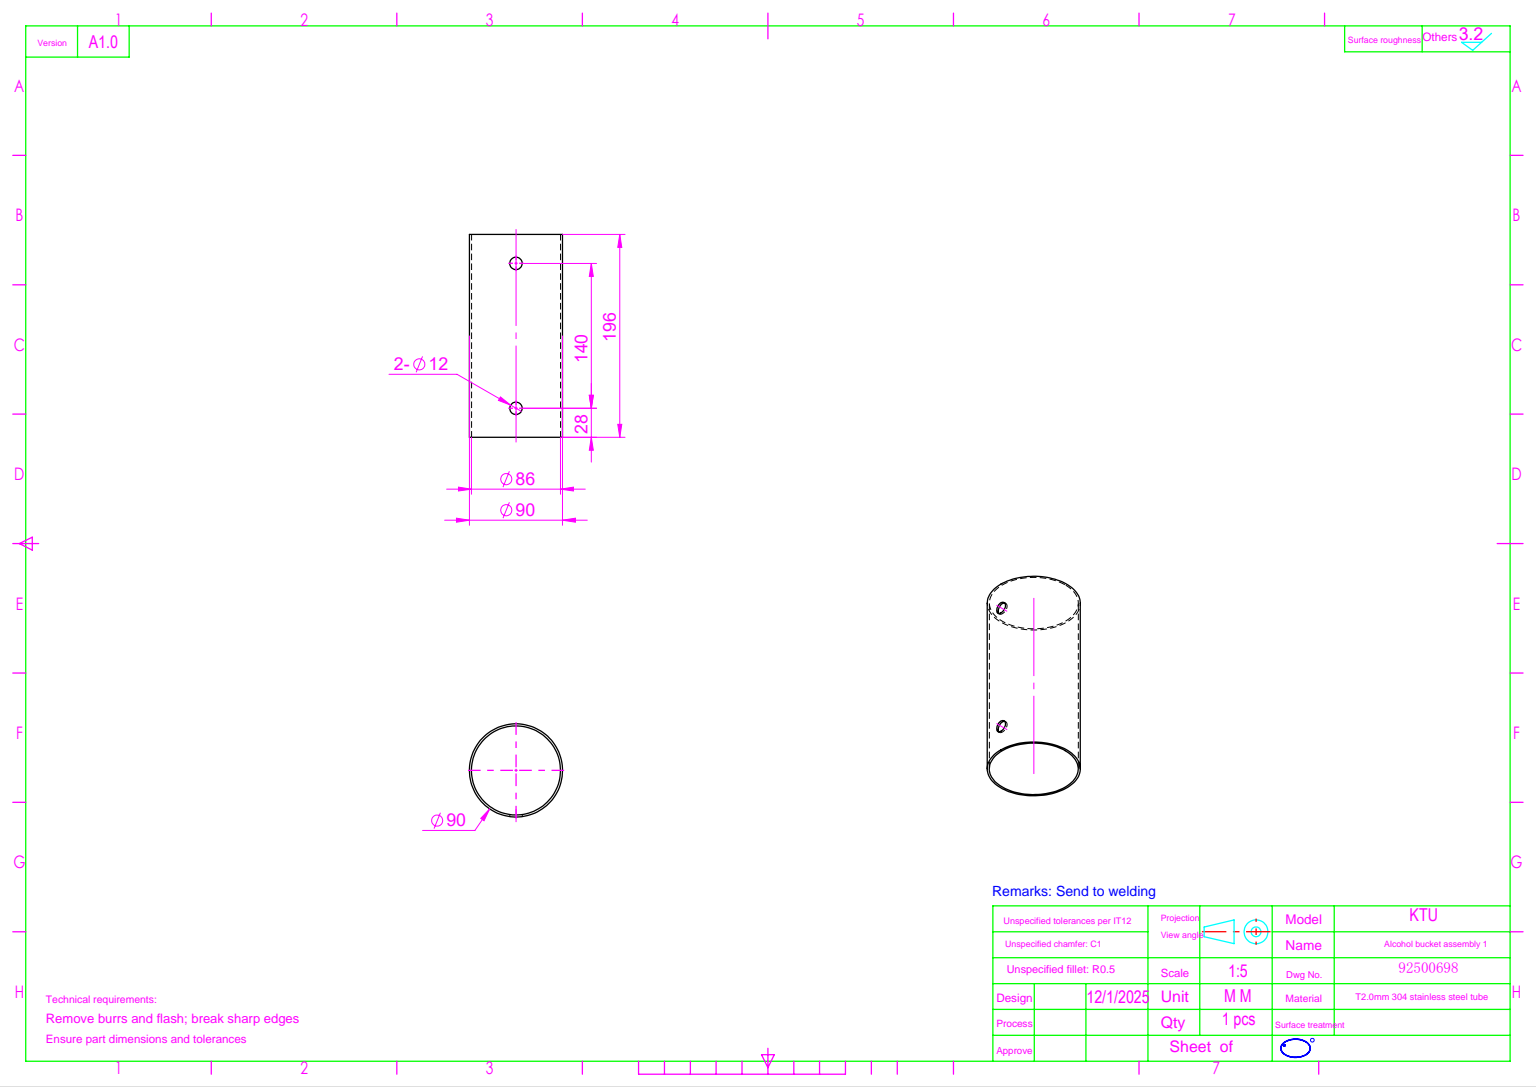
SolidWorks part; units mm, degrees
ref_plane "前视基准面" through (0, 0, 0) normal (0, 0, 1) x (1, 0, 0)
ref_plane "上视基准面" through (0, 0, 0) normal (0, 1, 0) x (1, 0, 0)
ref_plane "右视基准面" through (0, 0, 0) normal (1, 0, 0) x (0, 0, -1)
sketch "草图2" plane through (0, 0, 0) normal (0, 1, 0) x (1, 0, 0)
  circle A0 centre (0, 0) radius 45
  dimension "D1" = 90
extrude "拉伸-薄壁1" add sketch "草图2" along normal mid plane 196 thin thin type one direction reverse wall 2
sketch "草图3" plane through (0, 0, 0) normal (0, 0, 1) x (1, 0, 0)
  line L0 (-45, -98) -> (45, -98) construction
  circle A0 centre (0, 70) radius 6
  circle A1 centre (0, -70) radius 6
  dimension "D1" = 28
  dimension "D3" = 12
  dimension "D2" = 140
extrude "切除-拉伸2" cut sketch "草图3" along normal through all
